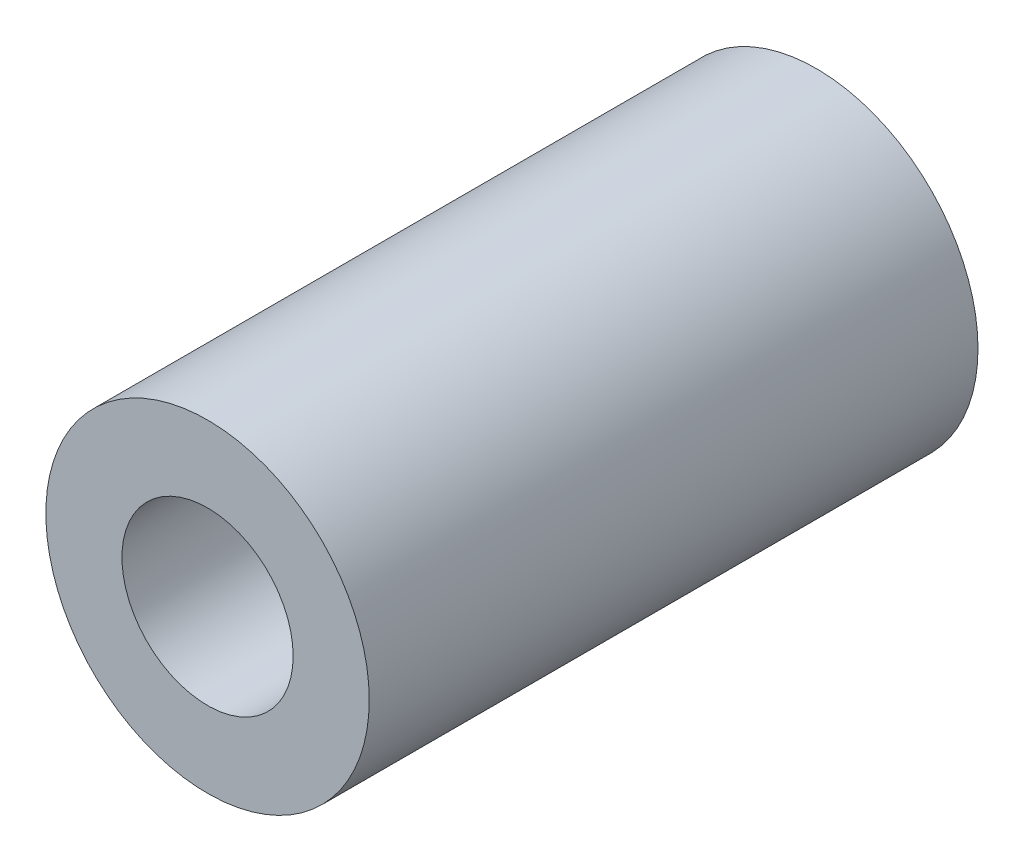
SolidWorks part; units mm, degrees
ref_plane "Front Plane" through (0, 0, 0) normal (0, 0, 1) x (1, 0, 0)
ref_plane "Top Plane" through (0, 0, 0) normal (0, 1, 0) x (1, 0, 0)
ref_plane "Right Plane" through (0, 0, 0) normal (1, 0, 0) x (0, 0, -1)
sketch "Sketch1" plane through (0, 0, 0) normal (0, 0, 1) x (1, 0, 0)
  circle A0 centre (0, 0) radius 4.5
  circle A1 centre (0, 0) radius 8.5
  dimension "D1" = 17
  dimension "D2" = 9
extrude "Boss-Extrude1" add sketch "Sketch1" along normal blind 32
